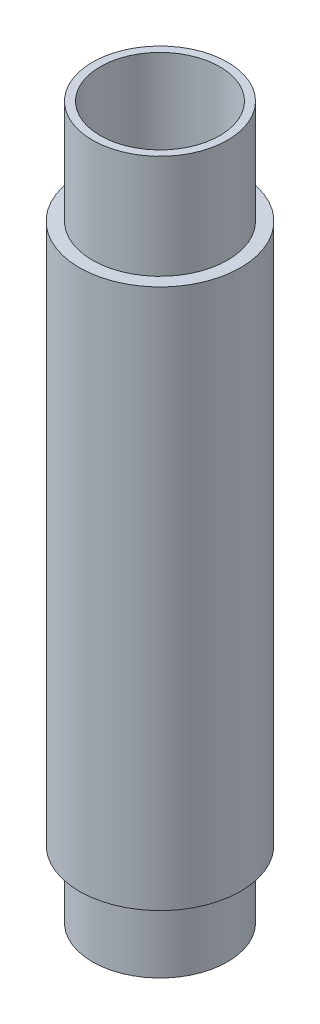
SolidWorks part; units mm, degrees
ref_plane "前视基准面" through (0, 0, 0) normal (0, 0, 1) x (1, 0, 0)
ref_plane "上视基准面" through (0, 0, 0) normal (0, 1, 0) x (1, 0, 0)
ref_plane "右视基准面" through (0, 0, 0) normal (1, 0, 0) x (0, 0, -1)
sketch "草图1" plane through (0, 0, 0) normal (0, 0, 1) x (1, 0, 0)
  line L0 (0, 125.6786) -> (0, -144.2976) construction
  line L1 (57.5, 470.0119) -> (57.5, -214.6181)
  line L2 (57.5, -214.6181) -> (65, -214.6181)
  line L3 (65, -214.6181) -> (65, -149.6181)
  line L4 (65, -149.6181) -> (77.5, -149.6181)
  line L5 (77.5, -149.6181) -> (77.5, 370.0119)
  line L6 (77.5, 370.0119) -> (65, 370.0119)
  line L7 (65, 370.0119) -> (65, 470.0119)
  line L8 (65, 470.0119) -> (57.5, 470.0119)
  dimension "D1" = 57.5
  dimension "D2" = 684.63
  dimension "D3" = 7.5
  dimension "D4" = 100
  dimension "D5" = 12.5
  dimension "D6" = 65
  dimension "D7" = 7.5
revolve "旋转1" add sketch "草图1" angle 360 about L0
